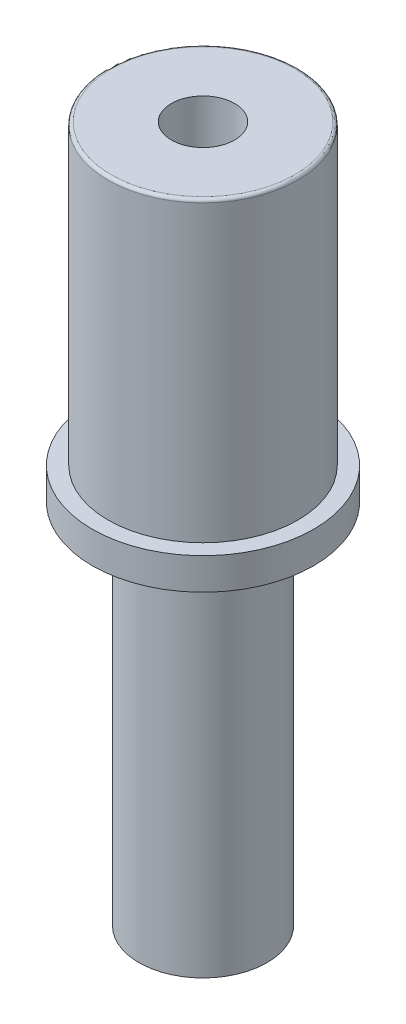
SolidWorks part; units mm, degrees
ref_plane "Front Plane" through (0, 0, 0) normal (0, 0, 1) x (1, 0, 0)
ref_plane "Top Plane" through (0, 0, 0) normal (0, 1, 0) x (1, 0, 0)
ref_plane "Right Plane" through (0, 0, 0) normal (1, 0, 0) x (0, 0, -1)
sketch "Sketch1" plane through (0, 0, 0) normal (0, 0, 1) x (1, 0, 0)
  line L0 (0, -19.747) -> (0, 23.2273) construction
  line L2 (-3.5, 0) -> (-2.0233, 0)
  line L3 (-3.5, 0) -> (-3.5, 1)
  line L4 (-3.5, 1) -> (-3, 1)
  line L6 (-1, 10.4) -> (-1, -11.6)
  line L7 (-1, -11.6) -> (-2.0233, -11.6)
  line L8 (-3, 1) -> (-3, 10.4)
  line L9 (-3, 10.4) -> (-1, 10.4)
  line L12 (-2.0233, 0) -> (-2.0233, -11.6)
  dimension "D1" = 1
  dimension "D2" = 7
  dimension "D4" = 1
  dimension "D5" = 11.6
  dimension "D6" = 0.5
revolve "Revolve1" add sketch "Sketch1" angle 360 about L0
fillet "Fillet3" radius 0.1 1 edges at (0, 10.4, -3)
